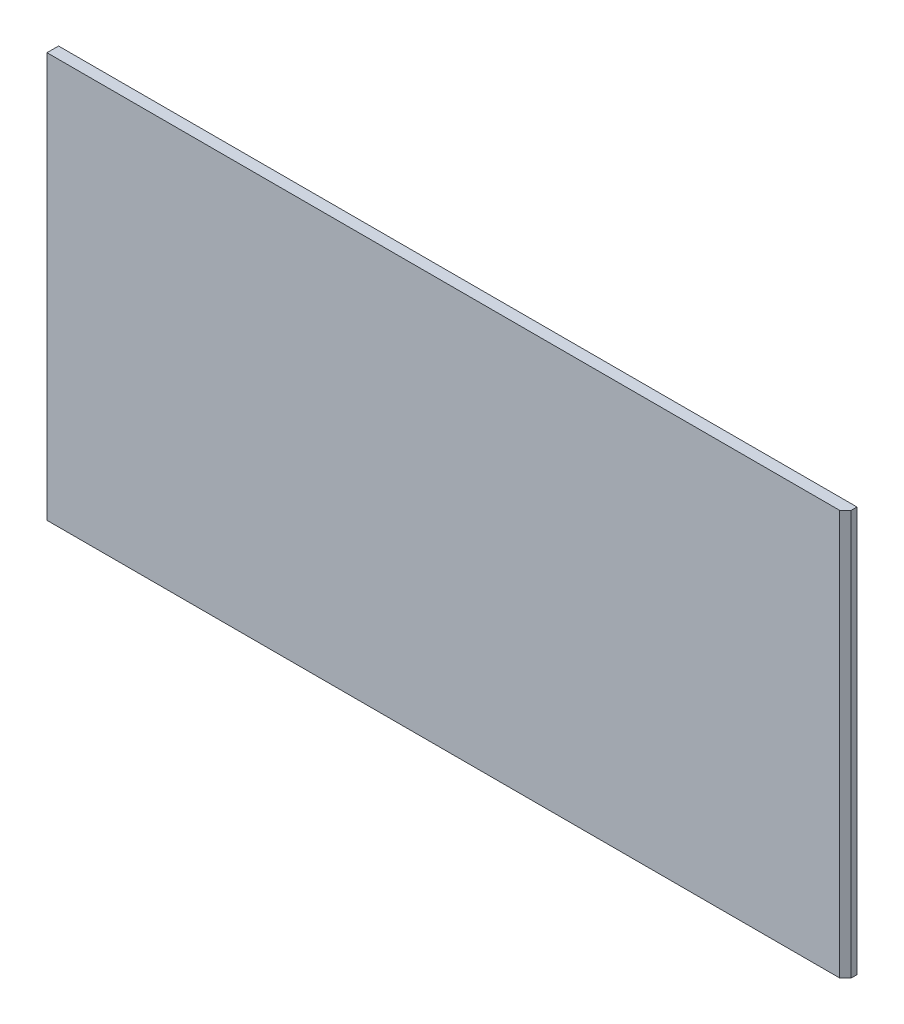
from build123d import *

# Parameters (mm, degrees)
SKETCH1_W           = 1380
SKETCH1_H           = 700
BOSS_EXTRUDE1_DEPTH = 20
CHAMFER1_SIZE       = 10


with BuildPart() as part:
    # Sketch1 → Boss-Extrude1 (new body)
    with BuildSketch(Plane.XY):
        with Locations((690, 350)):
            Rectangle(SKETCH1_W, SKETCH1_H)
    extrude(amount=BOSS_EXTRUDE1_DEPTH)

    # Chamfer1
    chamfer1_edges = [part.edges().sort_by_distance(p)[0] for p in [
        (1380, 350, 20),
    ]]
    chamfer(chamfer1_edges, length=CHAMFER1_SIZE)


solid = part.part
